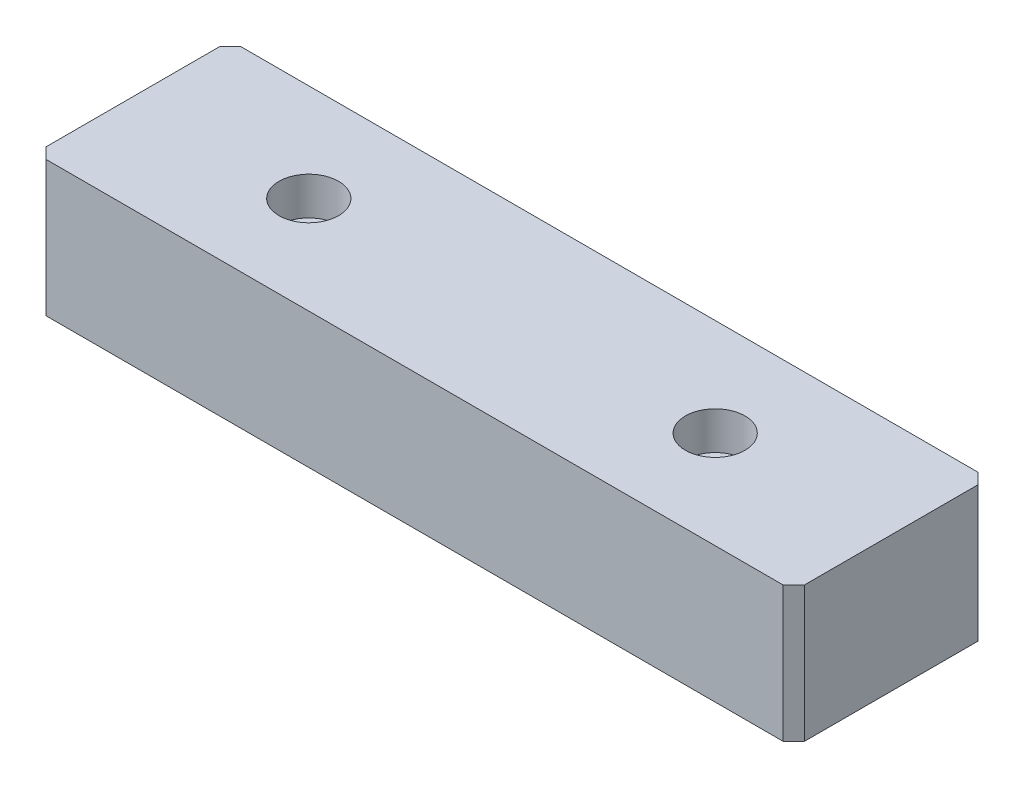
SolidWorks part; units mm, degrees
material "Q235A"
ref_plane "前视基准面" through (0, 0, 0) normal (0, 0, 1) x (1, 0, 0)
ref_plane "上视基准面" through (0, 0, 0) normal (0, 1, 0) x (1, 0, 0)
ref_plane "右视基准面" through (0, 0, 0) normal (1, 0, 0) x (0, 0, -1)
sketch "草图1" plane through (0, 0, 0) normal (0, 1, 0) x (1, 0, 0)
  line L1 (0, 0) -> (140, 0)
  line L2 (0, 0) -> (0, 36)
  line L3 (0, 36) -> (140, 36)
  line L4 (140, 0) -> (140, 36)
  dimension "D1" = 140
  dimension "D2" = 36
extrude "凸台-拉伸1" add sketch "草图1" along normal blind 25
hole_wizard "打孔尺寸(%根据)内六角圆柱头螺钉的类型1" positions "草图2" profile "草图3" counterbore size "M6" standard "GB" end condition through all
sketch "草图2" plane through (0, 25, 0) normal (0, 1, 0) x (1, 0, 0)
  line L0 (32.5, 18) -> (107.5, 18) construction
  line L2 (70, 36) -> (70, 18) construction
  line L3 (140, 36) -> (0, 36) construction
  line L5 (140, 18) -> (107.5, 18) construction
  line L6 (140, 0) -> (140, 36) construction
  point P0 (32.5, 18)
  point P2 (107.5, 18)
  dimension "D1" = 75
sketch "草图3" plane through (32.5, 25, -18) normal (1, 0, 0) x (0, 0, 1)
  line L0 (0, 0) -> (0, 25)
  line L1 (0, 25) -> (3.3, 25)
  line L3 (3.3, 25) -> (3.3, 7)
  line L4 (3.3, 7) -> (5.5, 7)
  line L5 (5.5, 7) -> (5.5, 0)
  line L7 (5.5, 0) -> (0, 0)
  line L11 (0, -6.35) -> (0, 107.95) construction
  dimension "通孔孔直径" = 6.6
  dimension "通孔孔深度" = 25
  dimension "柱形沉头孔直径" = 11
  dimension "柱形沉头孔深度" = 7
chamfer "倒角1" distance 2 angle 45 4 edges at (0, 12.5, -36) (0, 12.5, 0) (140, 12.5, -36) (140, 12.5, 0)
